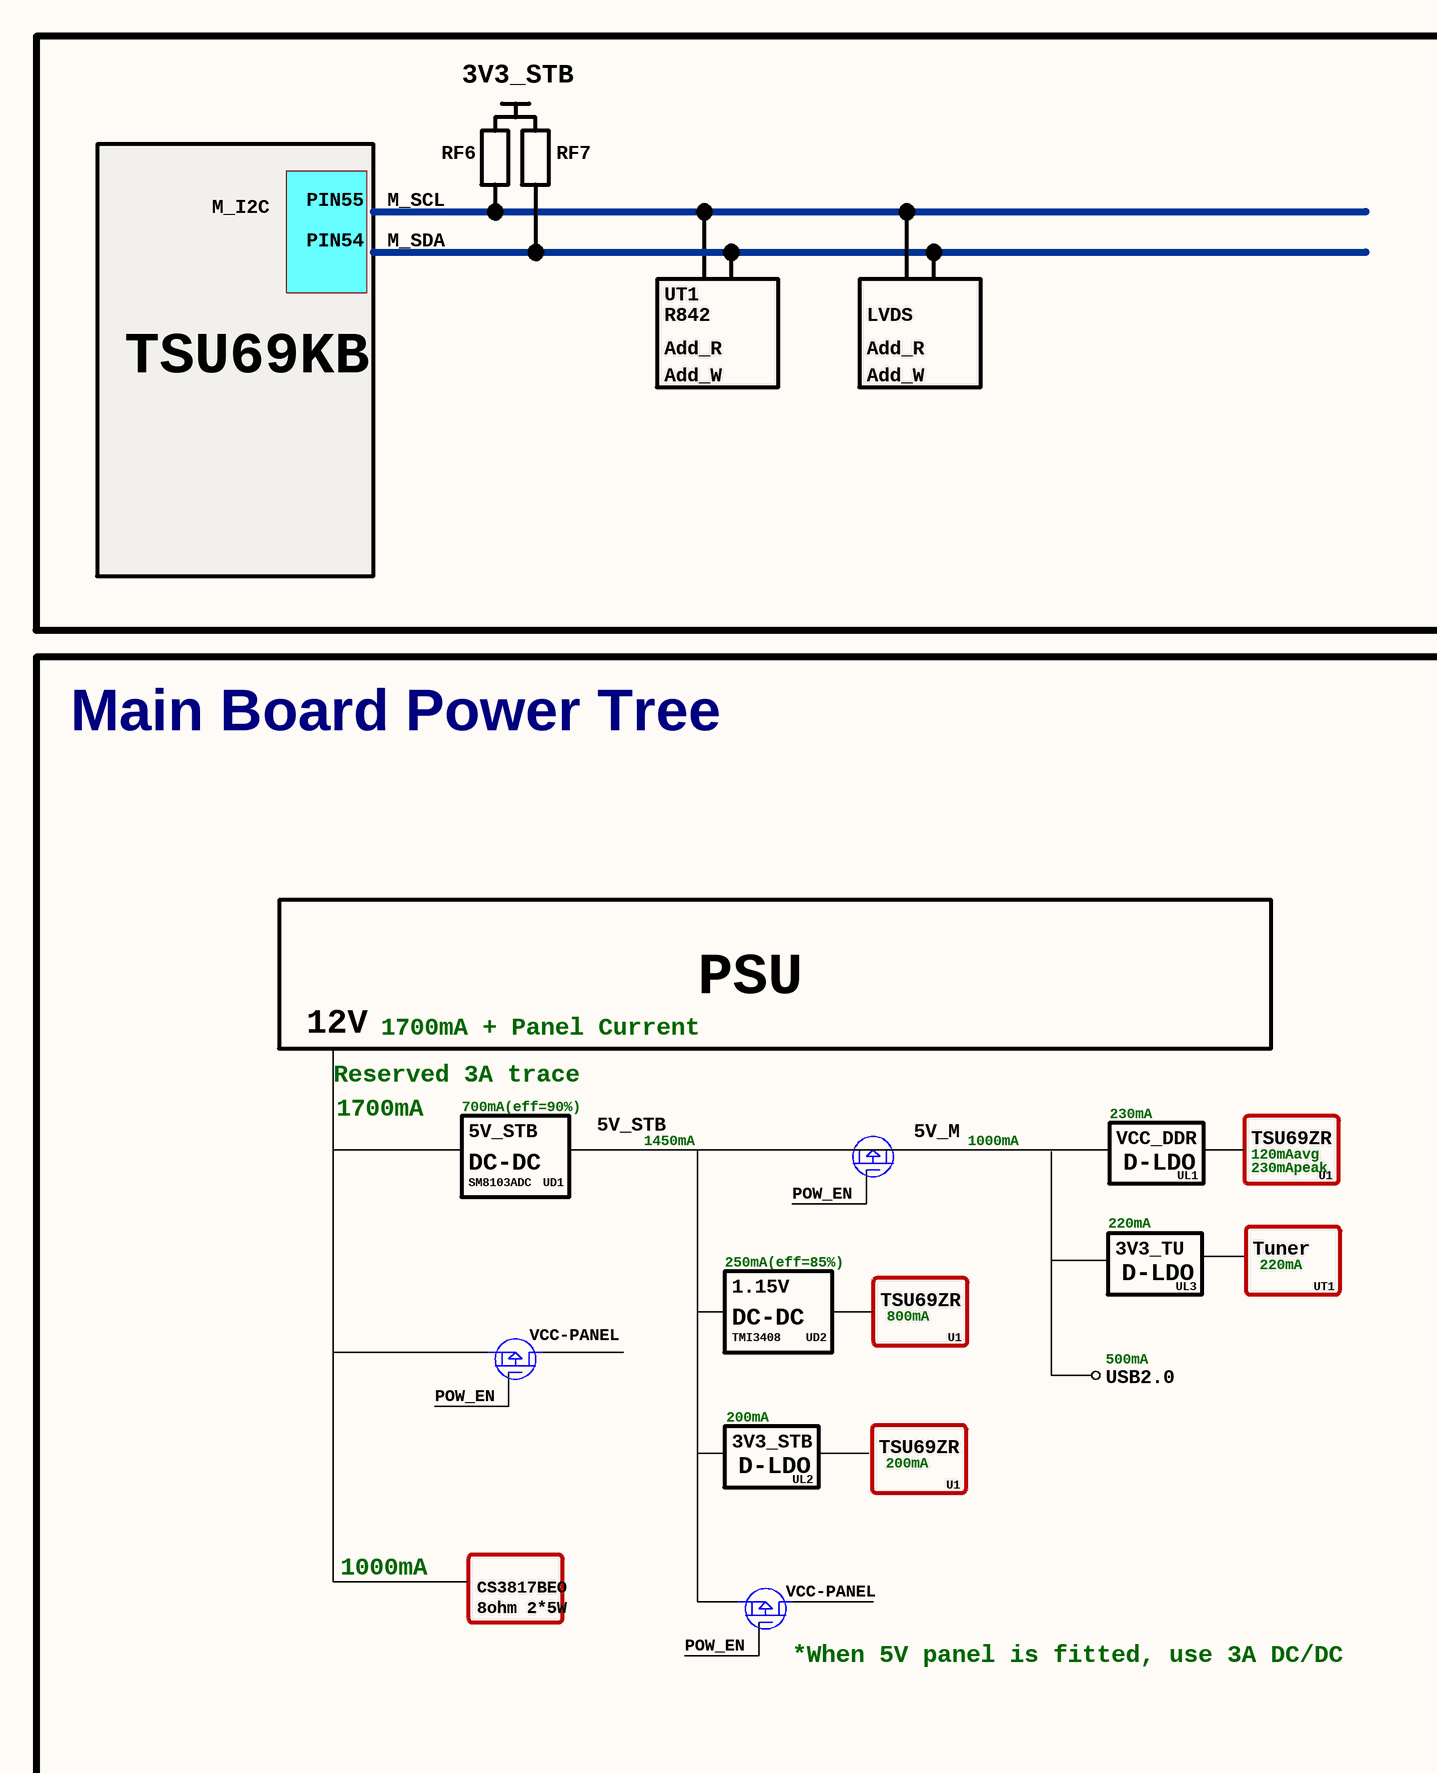
[diagram p0: MISC86383-10.SchDoc, left]
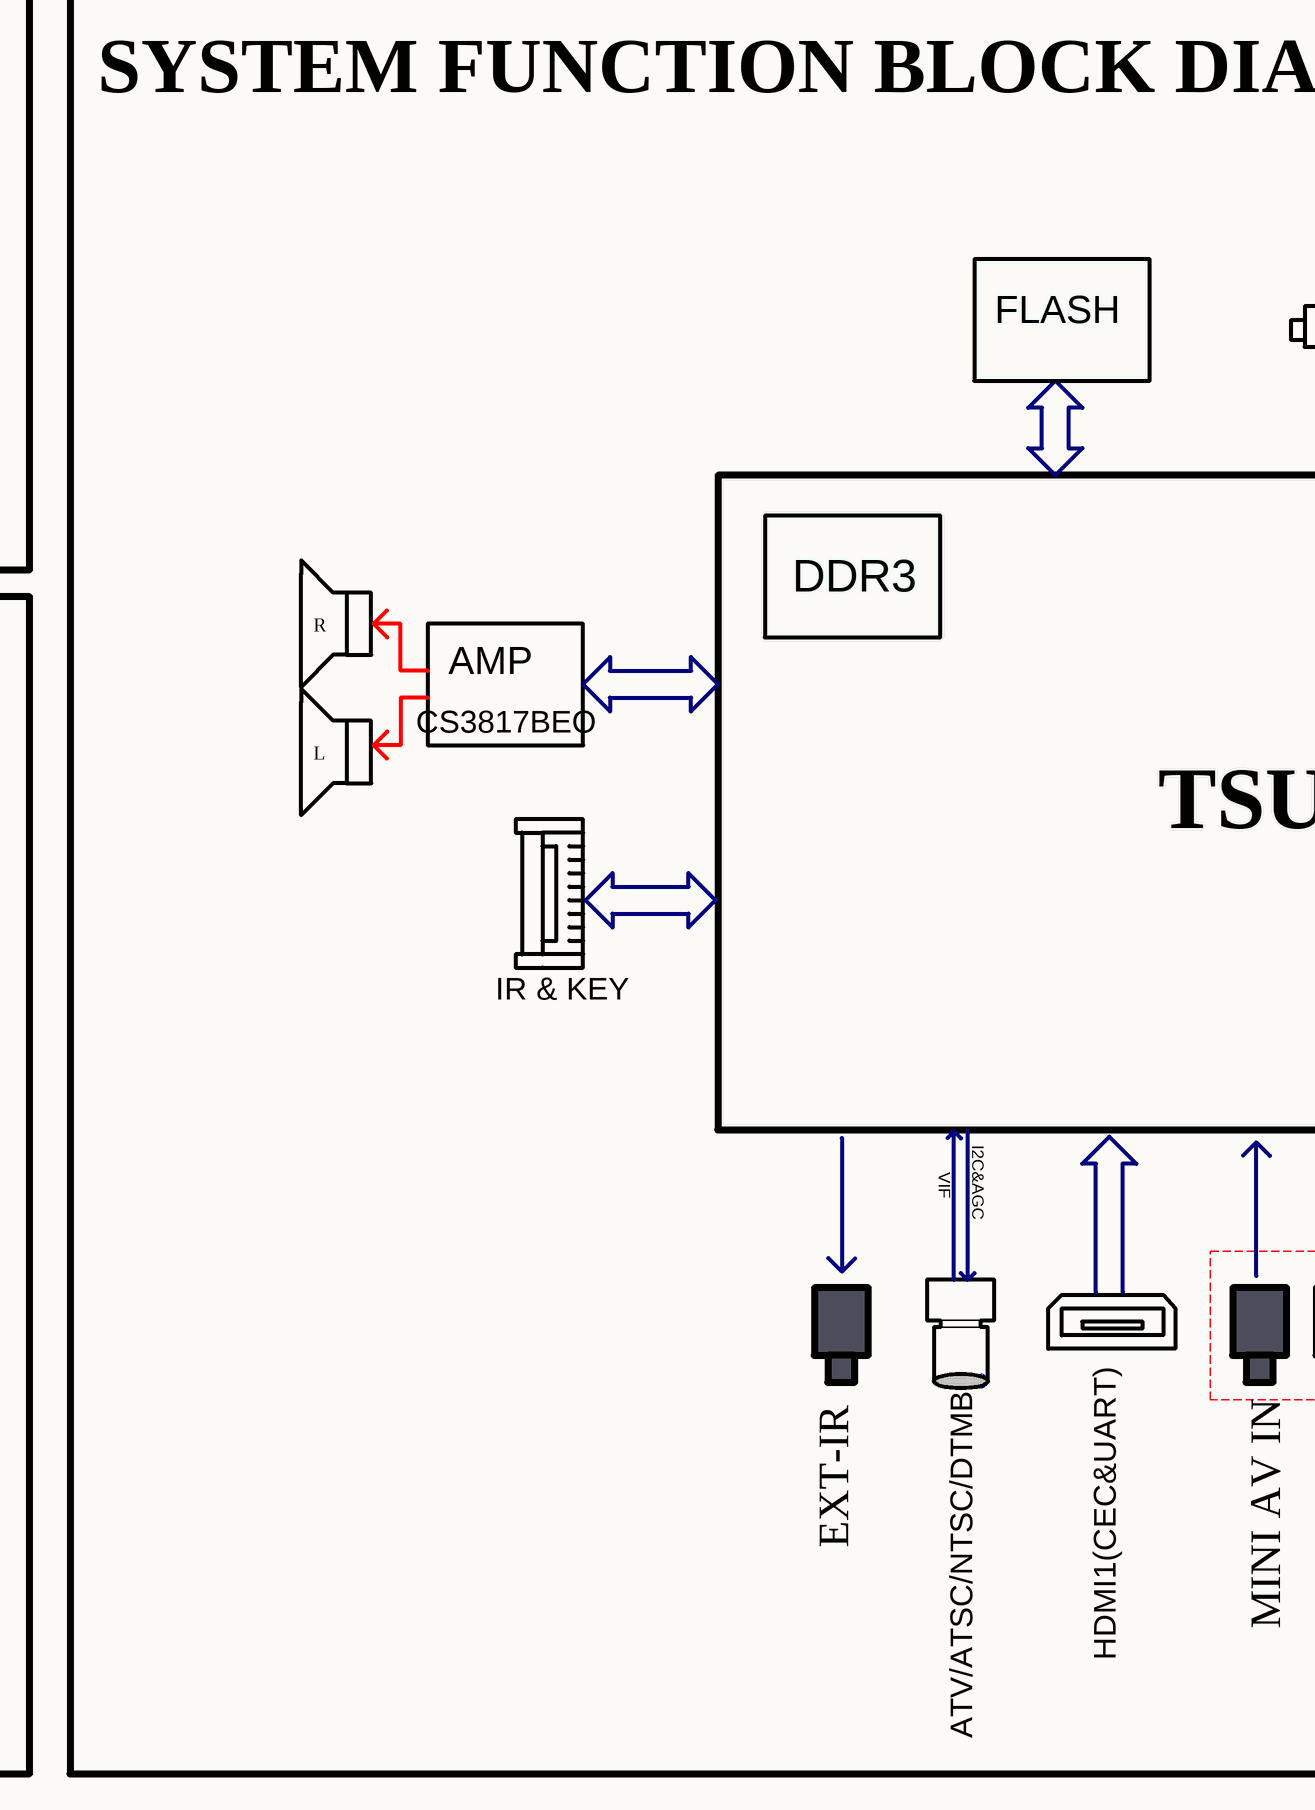
[diagram p1: MISC86383-10.SchDoc, middle]
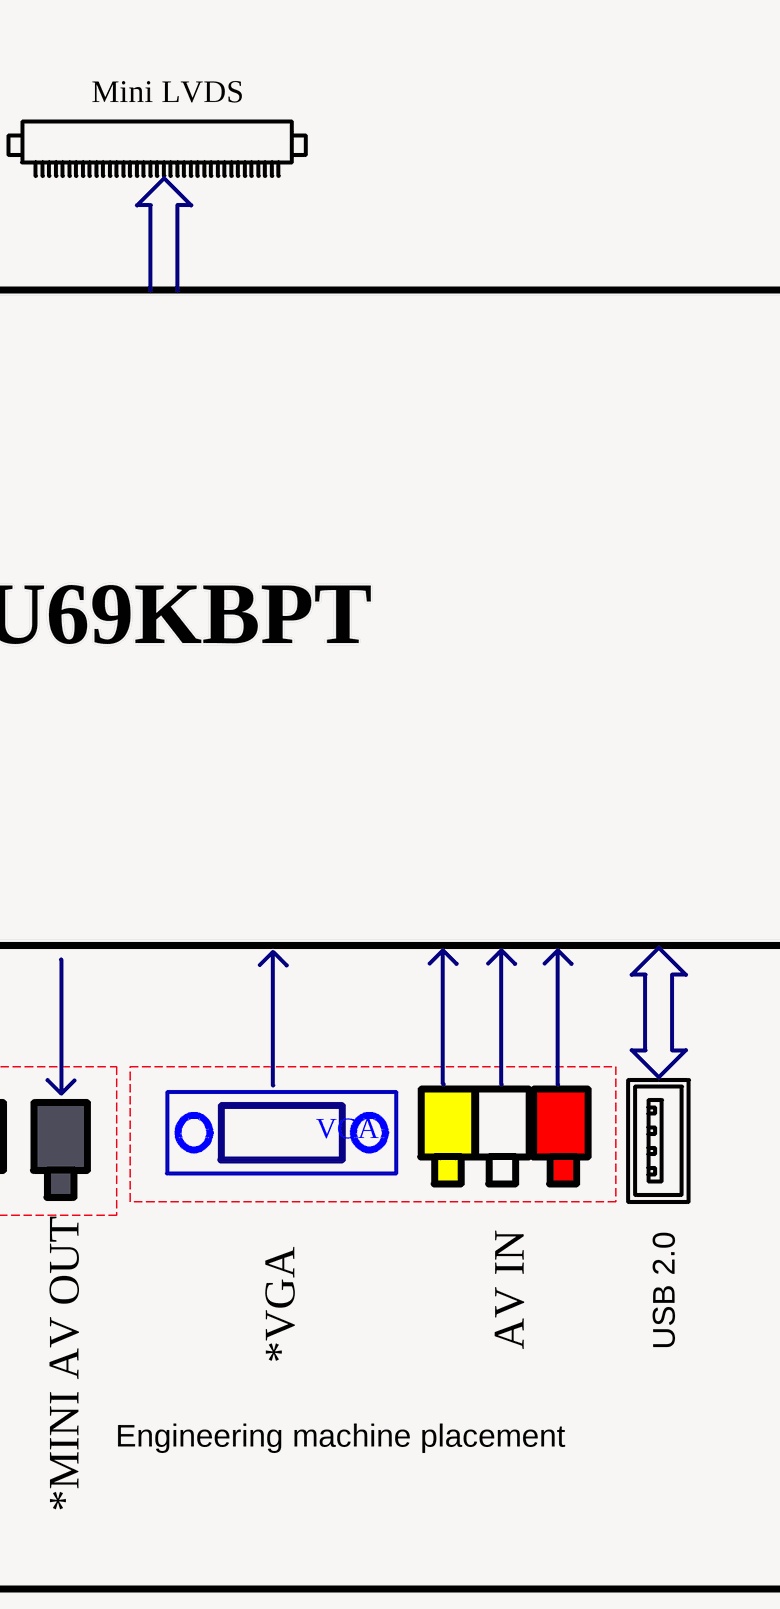
[diagram p2: MISC86383-10.SchDoc, right]
# Altium schematic sheet MISC86383-10.SchDoc
size 863 x 381 mm

## Parts
(Parts that share a designator on the sheet are numbered #1, #2 ... from top to bottom, then left to right.)
AV_IN  AV IN  (graphical)
MINI_AV#1  Name: EXT-IR  (hidden comment: MINI AV)  (graphical)
MINI_AV#2  Name: MINI AV IN  (hidden comment: MINI AV)  (graphical)
MINI_AV#3  Name: *MINI AV OUT  (hidden comment: MINI AV)  (graphical)
VGA  Name: *VGA  (hidden comment: VGA)  (graphical)

## Notes on the sheet
- 3V3_STB
- M_I2C
- PIN55
- M_SCL
- RF6
- RF7
- SYSTEM FUNCTION BLOCK DIAGRAM
- PIN54
- M_SDA
- UT1
- R842
- Add_R
- LVDS
- Mini LVDS
- TSU69KB
- Add_W
- FLASH
- R
- DDR3
- Main Board Power Tree
- AMP
- L
- CS3817BEO
- TSU69KBPT
- PSU
- 12V
- Reserved 3A trace
- 1700mA + Panel Current
- IR & KEY
- 1700mA
- 700mA(eff=90%)
- 5V_STB
- 1450mA
- 5V_M
- 1000mA
- 230mA
- VCC_DDR
- TSU69ZR
- 120mAavg
- DC-DC
- SM8103ADC
- UD1
- POW_EN
- 220mA
- D-LDO
- UL1
- 230mApeak
- U1
- VIF
- I2C&AGC
- 250mA(eff=85%)
- 1.15V
- 3V3_TU
- UL3
- Tuner
- VCC-PANEL
- TMI3408
- UD2
- 800mA
- 500mA
- 200mA
- USB2.0
- UL2
- 8ohm 2*5W
- USB 2.0
- *When 5V panel is fitted, use 3A DC/DC
- Engineering machine placement
- HDMI1(CEC&UART)
- ATV/ATSC/NTSC/DTMB

## Library data of the parts
AV_IN = AV IN: Name: AV IN